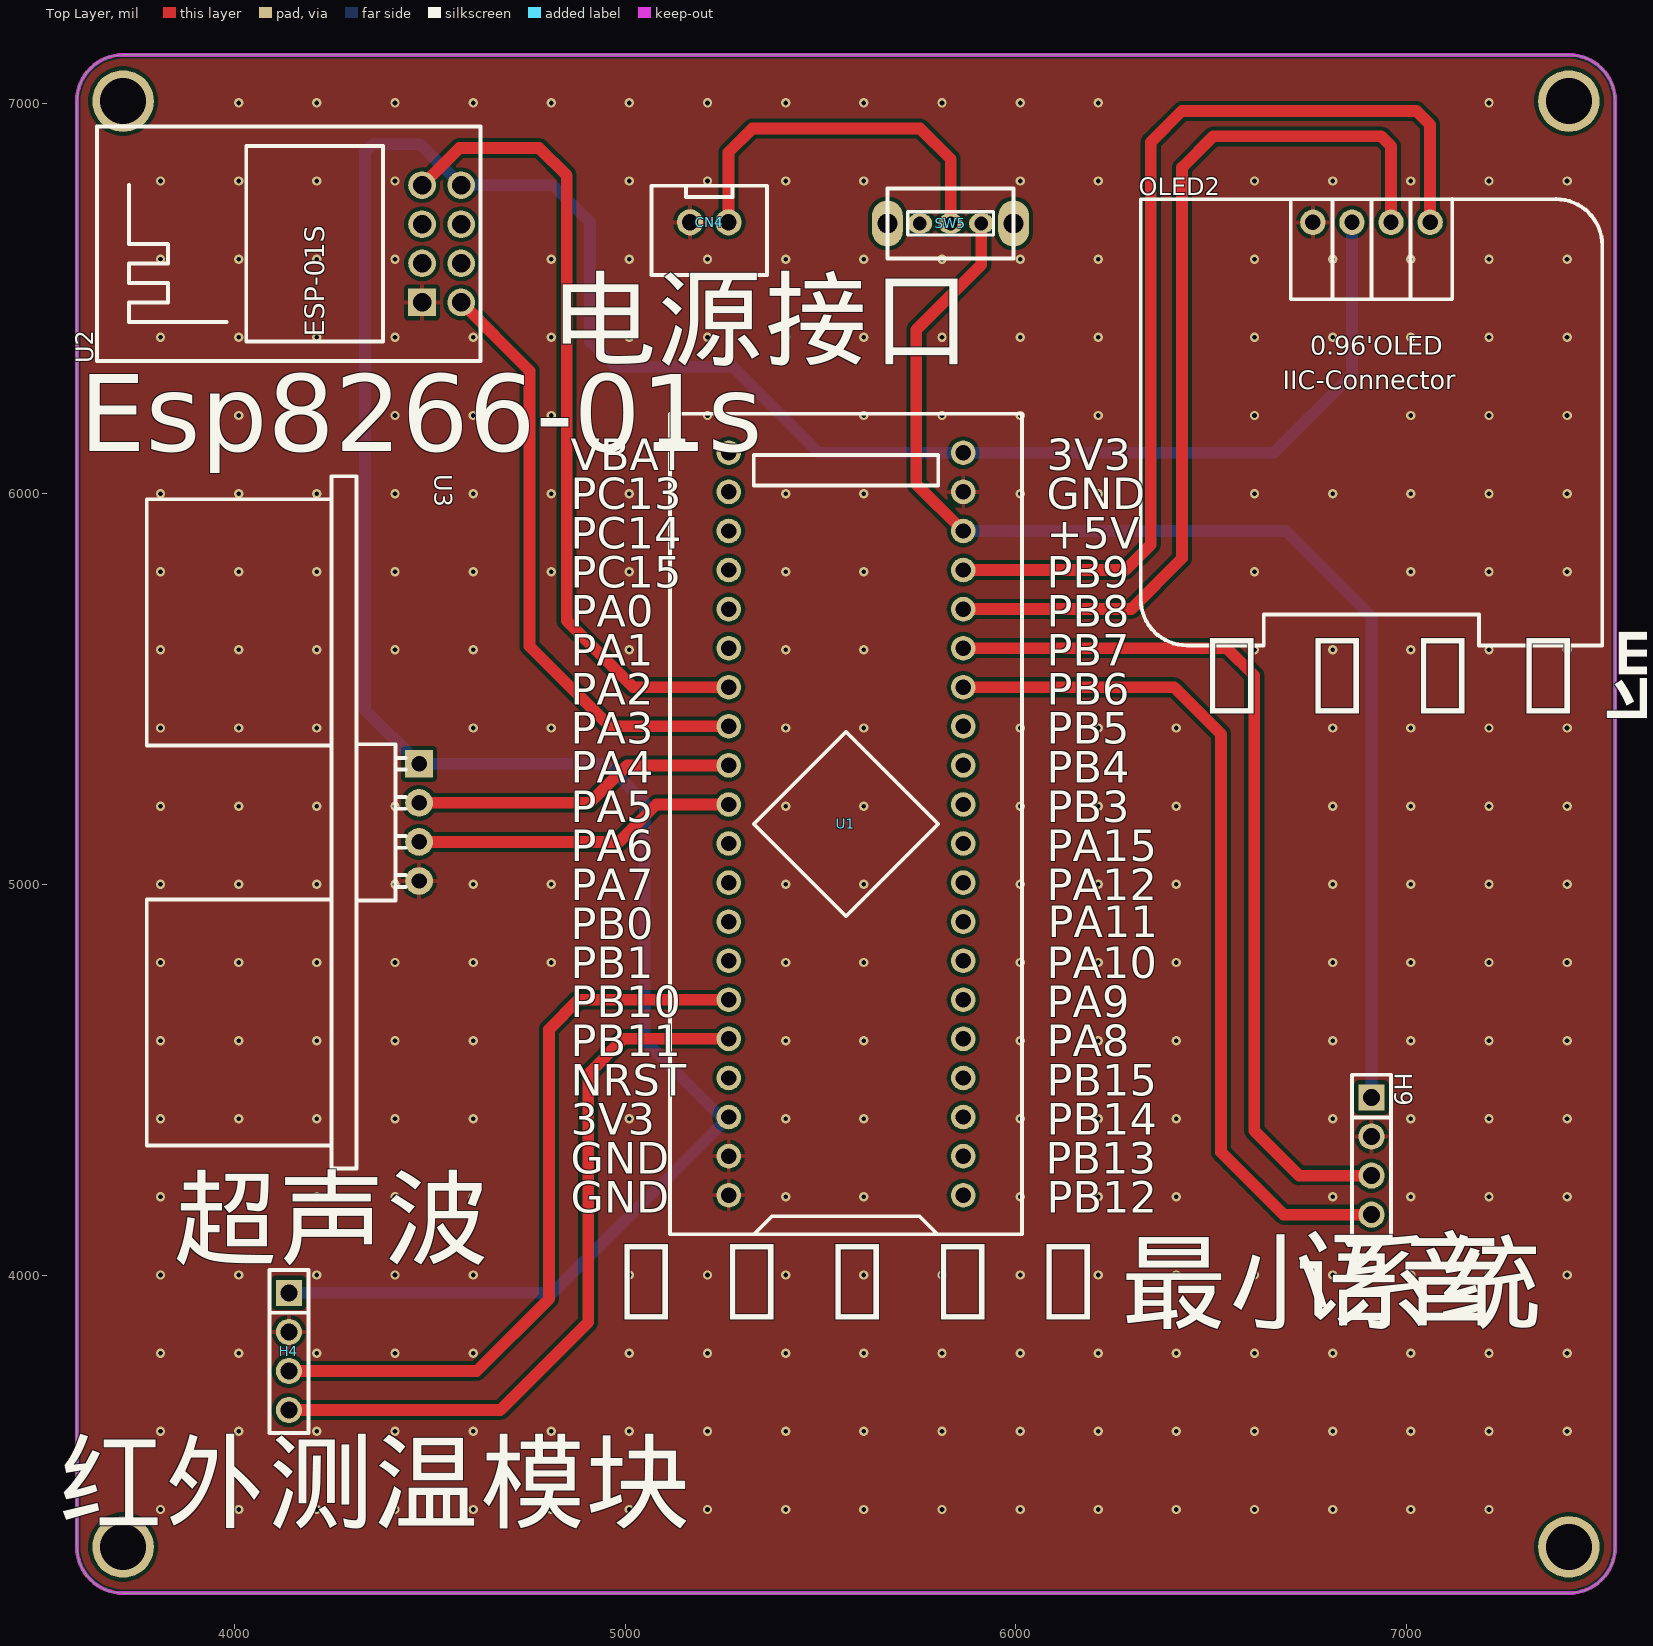
[diagram p0: Top Layer view]
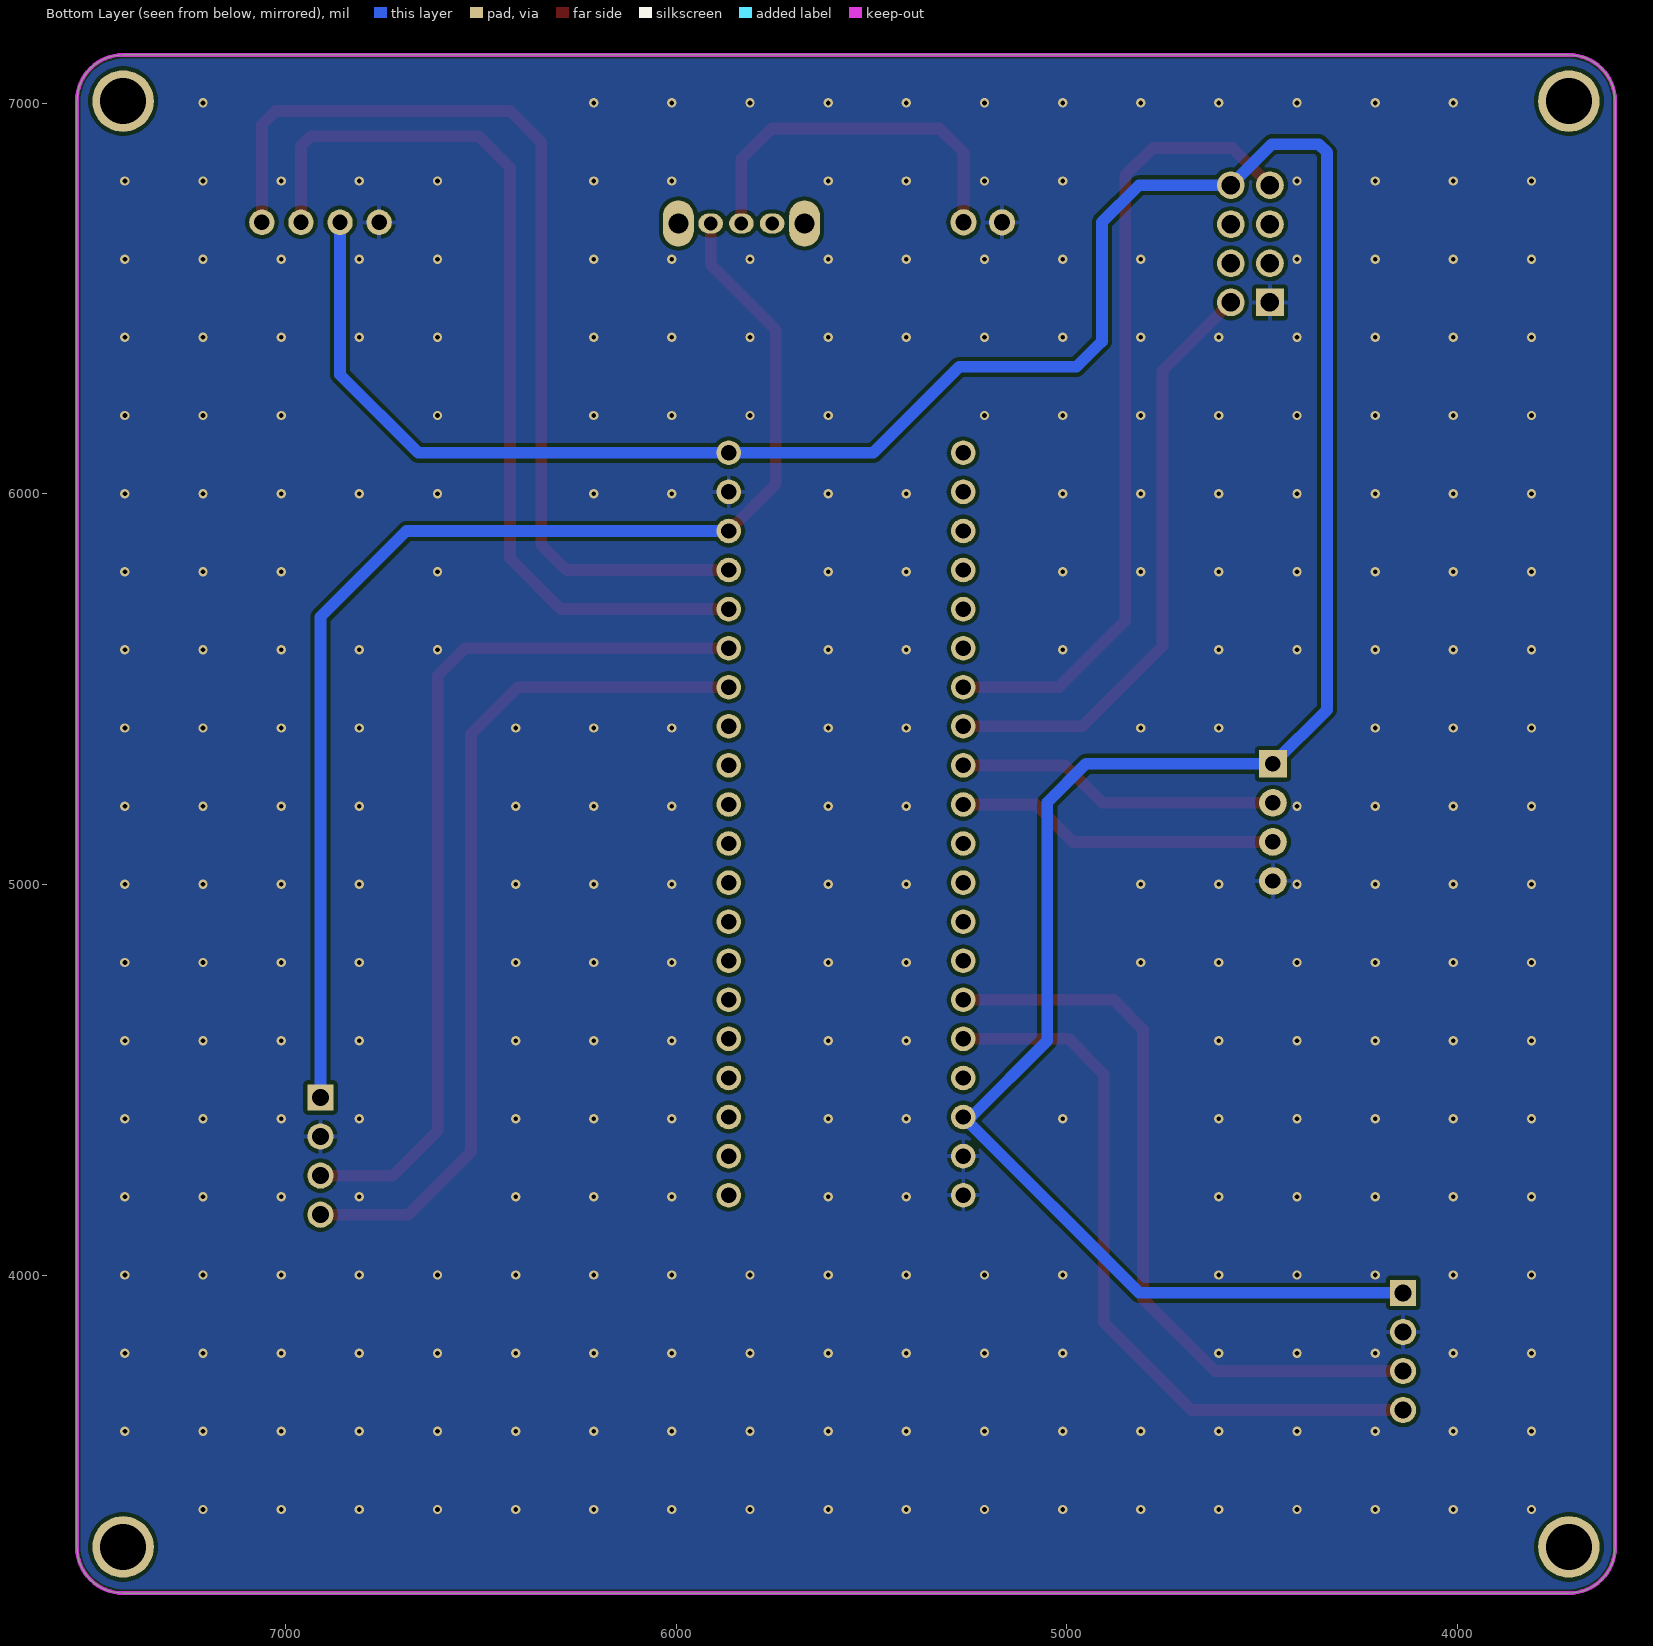
[diagram p1: Bottom Layer view, seen from below]
# Altium PCB MISC51851.pcbdoc
Units mil, origin at the board's own origin, x right, y up, seen from the top; angles counter-clockwise.
Board outline 3937.01 x 3937.01 mil, 2 copper layers (Top Layer, Bottom Layer), stack 62.206 mil thick; 8 components, 38 nets, 75 pads, 294 vias.

## Layer stack, top to bottom
Top Solder Mask Layer: solder mask 0.394, Dk 3.3
Top Layer: signal copper 1.379
Dielectric1: surface 59.449, FR4, Dk 4.5
Bottom Layer: signal copper 1.378
Bottom Solder Mask Layer: solder mask 0.394, Dk 3.3

## Board outline
3714.61,7123.5 ccw(c3714.61,7005.39) 3596.5,7005.39 3596.5,3304.61 ccw(c3714.61,3304.61) 3714.61,3186.5 7415.39,3186.5 ccw(c7415.39,3304.61) 7533.5,3304.61 7533.5,7005.39 ccw(c7415.39,7005.39) 7415.39,7123.5 3714.61,7123.5

## Design rules (kind name [scope] priority, off if disabled: settings)
BoardOutlineClearance copperThickness2oz_1 [All] p2 off: genericclearance=7.99 ignorepadtopadclearanceinfootprint=FALSE except(0: Arc-SplitContinuation Track-SplitContinuation SMDPad-SplitContinuation THPad-SplitContinuation Via-SplitContinuation Fill-SplitContinuation Region-SplitContinuation Poly-SplitContinuation Text-SplitContinuation Hole-SplitContinuation; 5.98: Arc-CutoutEdge Track-CutoutEdge SMDPad-CutoutEdge THPad-CutoutEdge Via-CutoutEdge Text-CutoutEdge; 6.9: Hole-OutlineEdge Hole-CutoutEdge; 10: Poly-OutlineEdge Poly-CutoutEdge; 11.81: Arc-OutlineEdge Track-OutlineEdge SMDPad-OutlineEdge THPad-OutlineEdge Via-OutlineEdge Fill-OutlineEdge Region-OutlineEdge Text-OutlineEdge Fill-CutoutEdge Region-CutoutEdge)
BoardOutlineClearance Plane_innerPlane_1 [All] p4 off: genericclearance=4.02 ignorepadtopadclearanceinfootprint=FALSE except(0: Arc-SplitContinuation Track-SplitContinuation SMDPad-SplitContinuation THPad-SplitContinuation Via-SplitContinuation Fill-SplitContinuation Region-SplitContinuation Poly-SplitContinuation Text-SplitContinuation Hole-SplitContinuation; 5.98: Arc-CutoutEdge Track-CutoutEdge SMDPad-CutoutEdge THPad-CutoutEdge Via-CutoutEdge Text-CutoutEdge; 6.9: Hole-OutlineEdge Hole-CutoutEdge; 10: Poly-OutlineEdge Poly-CutoutEdge; 11.81: Arc-OutlineEdge Track-OutlineEdge SMDPad-OutlineEdge THPad-OutlineEdge Via-OutlineEdge Fill-OutlineEdge Region-OutlineEdge Text-OutlineEdge Fill-CutoutEdge Region-CutoutEdge)
BoardOutlineClearance Copper_copperRegion_1 [All] p6 off: genericclearance=4.02 ignorepadtopadclearanceinfootprint=FALSE except(0: Arc-SplitContinuation Track-SplitContinuation SMDPad-SplitContinuation THPad-SplitContinuation Via-SplitContinuation Fill-SplitContinuation Region-SplitContinuation Poly-SplitContinuation Text-SplitContinuation Hole-SplitContinuation; 5.98: Arc-CutoutEdge Track-CutoutEdge SMDPad-CutoutEdge THPad-CutoutEdge Via-CutoutEdge Text-CutoutEdge; 6.9: Hole-OutlineEdge Hole-CutoutEdge; 10: Poly-OutlineEdge Poly-CutoutEdge; 11.81: Arc-OutlineEdge Track-OutlineEdge SMDPad-OutlineEdge THPad-OutlineEdge Via-OutlineEdge Fill-OutlineEdge Region-OutlineEdge Text-OutlineEdge Fill-CutoutEdge Region-CutoutEdge)
BoardOutlineClearance Copper_copperRegion_copperThickness1oz_1 [All] p8 off: genericclearance=4.02 ignorepadtopadclearanceinfootprint=FALSE except(0: Arc-SplitContinuation Track-SplitContinuation SMDPad-SplitContinuation THPad-SplitContinuation Via-SplitContinuation Fill-SplitContinuation Region-SplitContinuation Poly-SplitContinuation Text-SplitContinuation Hole-SplitContinuation; 5.98: Arc-CutoutEdge Track-CutoutEdge SMDPad-CutoutEdge THPad-CutoutEdge Via-CutoutEdge Text-CutoutEdge; 6.9: Hole-OutlineEdge Hole-CutoutEdge; 10: Poly-OutlineEdge Poly-CutoutEdge; 11.81: Arc-OutlineEdge Track-OutlineEdge SMDPad-OutlineEdge THPad-OutlineEdge Via-OutlineEdge Fill-OutlineEdge Region-OutlineEdge Text-OutlineEdge Fill-CutoutEdge Region-CutoutEdge)
BoardOutlineClearance Copper_copperRegion_Copper_copperRegion_1 [All] p10 off: genericclearance=4.02 ignorepadtopadclearanceinfootprint=FALSE except(0: Arc-SplitContinuation Track-SplitContinuation SMDPad-SplitContinuation THPad-SplitContinuation Via-SplitContinuation Fill-SplitContinuation Region-SplitContinuation Poly-SplitContinuation Text-SplitContinuation Hole-SplitContinuation; 5.98: Arc-CutoutEdge Track-CutoutEdge SMDPad-CutoutEdge THPad-CutoutEdge Via-CutoutEdge Text-CutoutEdge; 6.9: Hole-OutlineEdge Hole-CutoutEdge; 10: Poly-OutlineEdge Poly-CutoutEdge; 11.81: Arc-OutlineEdge Track-OutlineEdge SMDPad-OutlineEdge THPad-OutlineEdge Via-OutlineEdge Fill-OutlineEdge Region-OutlineEdge Text-OutlineEdge Fill-CutoutEdge Region-CutoutEdge)
BoardOutlineClearance copperThickness1oz_1 [All] p12: genericclearance=4.02 ignorepadtopadclearanceinfootprint=FALSE except(0: Arc-SplitContinuation Track-SplitContinuation SMDPad-SplitContinuation THPad-SplitContinuation Via-SplitContinuation Fill-SplitContinuation Region-SplitContinuation Poly-SplitContinuation Text-SplitContinuation Hole-SplitContinuation; 5.98: Arc-CutoutEdge Track-CutoutEdge SMDPad-CutoutEdge THPad-CutoutEdge Via-CutoutEdge Text-CutoutEdge; 6.9: Hole-OutlineEdge Hole-CutoutEdge; 10: Poly-OutlineEdge Poly-CutoutEdge; 11.81: Arc-OutlineEdge Track-OutlineEdge SMDPad-OutlineEdge THPad-OutlineEdge Via-OutlineEdge Fill-OutlineEdge Region-OutlineEdge Text-OutlineEdge Fill-CutoutEdge Region-CutoutEdge)
Clearance copperThickness2oz [All] p1 off: gap=7.99 ignorepadtopadclearanceinfootprint=FALSE except(5.98: SMDPad-Track SMDPad-SMDPad THPad-Track SMDPad-THPad THPad-THPad Track-Via SMDPad-Via THPad-Via Via-Via Fill-SMDPad Region-SMDPad Fill-THPad Region-THPad Fill-Via Region-Via Fill-Fill Fill-Region Region-Region Arc-Track Arc-SMDPad Arc-THPad Arc-Via Fill-Arc Region-Arc Arc-Arc Text-Track SMDPad-Text Text-THPad Text-Via Fill-Text Region-Text Arc-Text Text-Text; 6.9: Hole-Track Hole-SMDPad Hole-THPad Hole-Via Fill-Hole Region-Hole Hole-Arc Hole-Text; 10: Poly-Track Poly-SMDPad Poly-THPad Poly-Via Poly-Fill Poly-Region Poly-Poly Poly-Arc Poly-Text Poly-Hole; 11.81: Fill-Track Region-Track)
Clearance Plane_innerPlane [All] p3 off: gap=4.02 ignorepadtopadclearanceinfootprint=FALSE except(5.98: SMDPad-Track SMDPad-SMDPad THPad-Track SMDPad-THPad THPad-THPad Track-Via SMDPad-Via THPad-Via Via-Via Fill-SMDPad Region-SMDPad Fill-THPad Region-THPad Fill-Via Region-Via Fill-Fill Fill-Region Region-Region Arc-Track Arc-SMDPad Arc-THPad Arc-Via Fill-Arc Region-Arc Arc-Arc Text-Track SMDPad-Text Text-THPad Text-Via Fill-Text Region-Text Arc-Text Text-Text; 6.9: Hole-Track Hole-SMDPad Hole-THPad Hole-Via Fill-Hole Region-Hole Hole-Arc Hole-Text; 10: Poly-Track Poly-SMDPad Poly-THPad Poly-Via Poly-Fill Poly-Region Poly-Poly Poly-Arc Poly-Text Poly-Hole; 11.81: Fill-Track Region-Track)
Clearance Copper_copperRegion [All] p5 off: gap=4.02 ignorepadtopadclearanceinfootprint=FALSE except(5.98: SMDPad-Track SMDPad-SMDPad THPad-Track SMDPad-THPad THPad-THPad Track-Via SMDPad-Via THPad-Via Via-Via Fill-SMDPad Region-SMDPad Fill-THPad Region-THPad Fill-Via Region-Via Fill-Fill Fill-Region Region-Region Arc-Track Arc-SMDPad Arc-THPad Arc-Via Fill-Arc Region-Arc Arc-Arc Text-Track SMDPad-Text Text-THPad Text-Via Fill-Text Region-Text Arc-Text Text-Text; 6.9: Hole-Track Hole-SMDPad Hole-THPad Hole-Via Fill-Hole Region-Hole Hole-Arc Hole-Text; 10: Poly-Track Poly-SMDPad Poly-THPad Poly-Via Poly-Fill Poly-Region Poly-Poly Poly-Arc Poly-Text Poly-Hole; 11.81: Fill-Track Region-Track)
Clearance Copper_copperRegion_copperThickness1oz [All] p7 off: gap=4.02 ignorepadtopadclearanceinfootprint=FALSE except(5.98: SMDPad-Track SMDPad-SMDPad THPad-Track SMDPad-THPad THPad-THPad Track-Via SMDPad-Via THPad-Via Via-Via Fill-SMDPad Region-SMDPad Fill-THPad Region-THPad Fill-Via Region-Via Fill-Fill Fill-Region Region-Region Arc-Track Arc-SMDPad Arc-THPad Arc-Via Fill-Arc Region-Arc Arc-Arc Text-Track SMDPad-Text Text-THPad Text-Via Fill-Text Region-Text Arc-Text Text-Text; 6.9: Hole-Track Hole-SMDPad Hole-THPad Hole-Via Fill-Hole Region-Hole Hole-Arc Hole-Text; 10: Poly-Track Poly-SMDPad Poly-THPad Poly-Via Poly-Fill Poly-Region Poly-Poly Poly-Arc Poly-Text Poly-Hole; 11.81: Fill-Track Region-Track)
Clearance Copper_copperRegion_Copper_copperRegion [All] p9 off: gap=4.02 ignorepadtopadclearanceinfootprint=FALSE except(5.98: SMDPad-Track SMDPad-SMDPad THPad-Track SMDPad-THPad THPad-THPad Track-Via SMDPad-Via THPad-Via Via-Via Fill-SMDPad Region-SMDPad Fill-THPad Region-THPad Fill-Via Region-Via Fill-Fill Fill-Region Region-Region Arc-Track Arc-SMDPad Arc-THPad Arc-Via Fill-Arc Region-Arc Arc-Arc Text-Track SMDPad-Text Text-THPad Text-Via Fill-Text Region-Text Arc-Text Text-Text; 6.9: Hole-Track Hole-SMDPad Hole-THPad Hole-Via Fill-Hole Region-Hole Hole-Arc Hole-Text; 10: Poly-Track Poly-SMDPad Poly-THPad Poly-Via Poly-Fill Poly-Region Poly-Poly Poly-Arc Poly-Text Poly-Hole; 11.81: Fill-Track Region-Track)
Clearance copperThickness1oz [All] p11: gap=4.02 ignorepadtopadclearanceinfootprint=FALSE except(5.98: SMDPad-Track SMDPad-SMDPad THPad-Track SMDPad-THPad THPad-THPad Track-Via SMDPad-Via THPad-Via Via-Via Fill-SMDPad Region-SMDPad Fill-THPad Region-THPad Fill-Via Region-Via Fill-Fill Fill-Region Region-Region Arc-Track Arc-SMDPad Arc-THPad Arc-Via Fill-Arc Region-Arc Arc-Arc Text-Track SMDPad-Text Text-THPad Text-Via Fill-Text Region-Text Arc-Text Text-Text; 6.9: Hole-Track Hole-SMDPad Hole-THPad Hole-Via Fill-Hole Region-Hole Hole-Arc Hole-Text; 10: Poly-Track Poly-SMDPad Poly-THPad Poly-Via Poly-Fill Poly-Region Poly-Poly Poly-Arc Poly-Text Poly-Hole; 11.81: Fill-Track Region-Track)
DiffPairsRouting differentialPair [All] p1: maxlimit=6 minlimit=6 mostfreqgap=6 toplayer_minwidth=5 toplayer_prefwidth=10 toplayer_maxwidth=100 toplayer_mingap=6 toplayer_prefgap=6 toplayer_maxgap=6 bottomlayer_minwidth=5 bottomlayer_prefwidth=10 bottomlayer_maxwidth=100 bottomlayer_mingap=6 bottomlayer_prefgap=6 bottomlayer_maxgap=6 maxuncoupledlength=10
HoleToHoleClearance otherClearance [All] p1: gap=11.81 allowstackedmicrovias=TRUE
Length netLength [All] p1: minlimit=0 maxlimit=0
PasteMaskExpansion pasteMaskExpansion [All] p1: expansion=0
PlaneConnect innerPlane [All] p1: planeconnectstyle=Relief reliefexpansion=20 reliefentries=4 reliefconductorwidth=10 reliefairgap=10
PolygonConnect copperRegion_copperThickness1oz [All] p1 off: connectstyle=Relief reliefconductorwidth=10 reliefentries=4 polygonreliefangle="90 Angle" airgapwidth=10 via.connectstyle=Relief via.reliefconductorwidth=10 via.reliefentries=4 via.polygonreliefangle="90 Angle" via.airgapwidth=10
PolygonConnect copperRegion_Copper_copperRegion [All] p2 off: connectstyle=Relief reliefconductorwidth=10 reliefentries=4 polygonreliefangle="90 Angle" airgapwidth=10 via.connectstyle=Relief via.reliefconductorwidth=10 via.reliefentries=4 via.polygonreliefangle="90 Angle" via.airgapwidth=10
PolygonConnect copperRegion [All] p3: connectstyle=Relief reliefconductorwidth=10 reliefentries=4 polygonreliefangle="90 Angle" airgapwidth=10 via.connectstyle=Relief via.reliefconductorwidth=10 via.reliefentries=4 via.polygonreliefangle="90 Angle" via.airgapwidth=10
RoutingVias viaSize [All] p1: holewidth=12.01 width=24.02 viastyle="Through Hole" minholewidth=11.81 minwidth=19.68 maxholewidth=248.03 maxwidth=393.7
SolderMaskExpansion solderMaskExpansion [IsVia] p1: expansion=-1000 istentingtop=TRUE
SolderMaskExpansion solderMaskExpansion [All] p2: expansion=2 istentingtop=FALSE
Width copperThickness2oz_2 [All] p1 off: maxlimit=100 minlimit=8 preferedwidth=10
Width copperThickness1oz_2 [All] p2: maxlimit=100 minlimit=5 preferedwidth=10

## Components (designator, comment, footprint, x,y, rotation, side; value= is the part's Value field where it differs from the comment)
CN4 "XH2.54*2P_直插" CONN-TH_2P-P2.50-XH2.54-2P 5215,6695 r0 top
H4 "" HDR-TH_4P-P2.54-V-F 4139,3804.93 r270 top
H9 "" HDR-TH_4P-P2.54-V-F 6910,4305 r270 top
OLED2 "" 0.96OLED_4P 6910,6695 r0 top
SW5 "" 拨动开关 5837.9,6692.05 r180 top
U1 "STM32F103C8T6-Card" CONN-TH_L53.3-W22.9_STM32F103C8T6-CARD 5565,5155 r90 top
U2 "ESP-01S" WIFIM-TH_ESP-01S 4530,6640 r90 top
U3 "HC-SR04" TH_HC-SR04V 4472.28,5159.1 r270 top

## Footprints (in the part's own frame and the unit in brackets; to place one, negate y for a bottom-side part, rotate by r counter-clockwise, add the part's x,y. Pads: shape width x height; smd on the part's side, far side on the other; paste and mask are expansions set on the pad)
0.96OLED_4P [mm]
  round 1.65 hole 1 copper offset 0,0: 1(-3.81,-0.001) 2(-1.27,0.002) 3(1.27,0.002) 4(3.81,0.002)
  silkscreen extent -15,-27.5 15,1.5
CONN-TH_2P-P2.50-XH2.54-2P [mm]
  round 1.7 hole 1.05 paste+0 mask+0.05: 1(1.25,0) 2(-1.25,0)
  silkscreen extent -3.75,-3.42 3.75,2.37
CONN-TH_L53.3-W22.9_STM32F103C8T6-CARD [mm]
  round 1.6 hole 1: 1(-24.13,-7.62) 2(-21.59,-7.62) 3(-19.05,-7.62) 4(-16.51,-7.62) 5(-13.97,-7.62) 6(-11.43,-7.62) 7(-8.89,-7.62) 8(-6.35,-7.62) 9(-3.81,-7.62) 10(-1.27,-7.62) 11(1.27,-7.62) 12(3.81,-7.62) 13(6.35,-7.62) 14(8.89,-7.62) 15(11.43,-7.62) 16(13.97,-7.62) 17(16.51,-7.62) 18(19.05,-7.62) 19(21.59,-7.62) 20(24.13,-7.62) 21(24.13,7.62) 22(21.59,7.62) 23(19.05,7.62) 24(16.51,7.62) 25(13.97,7.62) 26(11.43,7.62) 27(8.89,7.62) 28(6.35,7.62) 29(3.81,7.62) 30(1.27,7.62) 31(-1.27,7.62) 32(-3.81,7.62) 33(-6.35,7.62) 34(-8.89,7.62) 35(-11.43,7.62) 36(-13.97,7.62) 37(-16.51,7.62) 38(-19.05,7.62) 39(-21.59,7.62) 40(-24.13,7.62)
  silkscreen extent -26.67,-11.43 26.67,11.43
HDR-TH_4P-P2.54-V-F [mm]
  rect 1.7x1.7 hole 1.1: 1(-3.81,0)
  round 1.7 hole 1.1: 2(-1.27,0) 3(1.27,0) 4(3.81,0)
  silkscreen extent -5.29,-1.27 5.29,1.27
TH_HC-SR04V [mm]
  rect 1.8x1.8 hole 1.001: 1(-3.81,0)
  round 1.8 hole 1.001: 2(-1.27,0) 3(1.27,0) 4(3.81,0)
  silkscreen extent -22.5,-17.7 22.5,-0.89
WIFIM-TH_ESP-01S [mm]
  rect 1.8x1.8 hole 1.2: 1(-3.81,1.27)
  round 1.8 hole 1.2: 2(-1.27,1.27) 3(1.27,1.27) 4(3.81,1.27) 5(3.81,-1.27) 6(1.27,-1.27) 7(-1.27,-1.27) 8(-3.81,-1.27)
  silkscreen extent -7.62,-2.54 7.62,22.4
拨动开关 [mil]
  oval 63x51.2 hole 35.4 paste+0 mask+2: 1(-73.4,0) 2(5,0) 3(84,0)
  oval 78.7x118.1 hole 51.2 paste+0 mask+2: 4(166.7,0) 5(-156.1,0)
  silkscreen extent -156,-90 167,90

## Free pads (board coordinates)
  round 157.48 hole 118.11: 1(3714.61,7005.39) 1(3714.61,3304.61) 1(7415.39,7005.39) 1(7415.39,3304.61)

## Via types
v1: diameter 24.02, hole 12, Top Layer to Bottom Layer, 294 vias

## Nets (pads, with @x,y where several pads share a name; then routed paths per layer and width w, separated by ;. In a path a pad name is that pad's centre, name@x,y a point inside that pad or via, vN(x,y) a via of type N, cw(c..) or ccw(c..) an arc to the next point about the centre after c; other vN are vias at no path point)
$1N17118: CN4.1 SW5.2 | length 970.4
  Top Layer w30: CN4.1 5264.22,6874.22 5325,6935 5755,6935 5832.9,6857.1 SW5.2
+5V: H9.1 SW5.1 U1.18 | length 3271.8
  Top Layer w30: U1.18 5745,6025 5745,6420 5911.3,6586.3 SW5.1
  Bottom Layer w30: U1.18 6690,5905 6910,5685 H9.1
GND: CN4.2 H4.2 H9.2 OLED2.1 U1.19 U1.39 U1.40 U2.1 U3.4
  other v1: 3810.6,3400.6 4010.6,3400.6 4210.6,3400.6 4410.6,3400.6 4610.6,3400.6 4810.6,3400.6 5010.6,3400.6 5210.6,3400.6 5410.6,3400.6 5610.6,3400.6 5810.6,3400.6 6010.6,3400.6 6210.6,3400.6 6410.6,3400.6 6610.6,3400.6 6810.6,3400.6 7010.6,3400.6 7210.6,3400.6 3810.6,3600.6 4010.6,3600.6 4210.6,3600.6 4410.6,3600.6 4610.6,3600.6 4810.6,3600.6 5010.6,3600.6 5210.6,3600.6 5410.6,3600.6 5610.6,3600.6 5810.6,3600.6 6010.6,3600.6 6210.6,3600.6 6410.6,3600.6 6610.6,3600.6 6810.6,3600.6 7010.6,3600.6 7210.6,3600.6 7410.6,3600.6 3810.6,3800.6 4010.6,3800.6 4210.6,3800.6 4410.6,3800.6 4610.6,3800.6 5010.6,3800.6 5210.6,3800.6 5410.6,3800.6 5610.6,3800.6 5810.6,3800.6 6010.6,3800.6 6210.6,3800.6 6410.6,3800.6 6610.6,3800.6 6810.6,3800.6 7010.6,3800.6 7210.6,3800.6 7410.6,3800.6 3810.6,4000.6 4010.6,4000.6 4210.6,4000.6 4410.6,4000.6 4610.6,4000.6 5010.6,4000.6 5210.6,4000.6 5410.6,4000.6 5610.6,4000.6 5810.6,4000.6 6010.6,4000.6 6210.6,4000.6 6410.6,4000.6 6610.6,4000.6 6810.6,4000.6 7010.6,4000.6 7210.6,4000.6 7410.6,4000.6 3810.6,4200.6 4010.6,4200.6 4210.6,4200.6 4410.6,4200.6 4610.6,4200.6 5410.6,4200.6 5610.6,4200.6 6010.6,4200.6 6210.6,4200.6 6410.6,4200.6 6810.6,4200.6 7010.6,4200.6 7210.6,4200.6 7410.6,4200.6 3810.6,4400.6 4010.6,4400.6 4210.6,4400.6 4410.6,4400.6 4610.6,4400.6 5010.6,4400.6 5410.6,4400.6 5610.6,4400.6 6010.6,4400.6 6210.6,4400.6 6410.6,4400.6 6810.6,4400.6 7010.6,4400.6 7210.6,4400.6 7410.6,4400.6 3810.6,4600.6 4010.6,4600.6 4210.6,4600.6 4410.6,4600.6 4610.6,4600.6 5410.6,4600.6 5610.6,4600.6 6010.6,4600.6 6210.6,4600.6 6410.6,4600.6 6810.6,4600.6 7010.6,4600.6 7210.6,4600.6 7410.6,4600.6 3810.6,4800.6 4010.6,4800.6 4210.6,4800.6 4410.6,4800.6 4610.6,4800.6 4810.6,4800.6 5410.6,4800.6 5610.6,4800.6 6010.6,4800.6 6210.6,4800.6 6410.6,4800.6 6810.6,4800.6 7010.6,4800.6 7210.6,4800.6 7410.6,4800.6 3810.6,5000.6 4010.6,5000.6 4210.6,5000.6 4410.6,5000.6 4610.6,5000.6 4810.6,5000.6 5410.6,5000.6 5610.6,5000.6 6010.6,5000.6 6210.6,5000.6 6410.6,5000.6 6810.6,5000.6 7010.6,5000.6 7210.6,5000.6 7410.6,5000.6 3810.6,5200.6 4010.6,5200.6 4210.6,5200.6 4410.6,5200.6 5410.6,5200.6 5610.6,5200.6 6010.6,5200.6 6210.6,5200.6 6410.6,5200.6 6810.6,5200.6 7010.6,5200.6 7210.6,5200.6 7410.6,5200.6 3810.6,5400.6 4010.6,5400.6 4210.6,5400.6 4610.6,5400.6 4810.6,5400.6 5410.6,5400.6 5610.6,5400.6 6010.6,5400.6 6210.6,5400.6 6410.6,5400.6 6810.6,5400.6 7010.6,5400.6 7210.6,5400.6 7410.6,5400.6 3810.6,5600.6 4010.6,5600.6 4210.6,5600.6 4410.6,5600.6 4610.6,5600.6 5010.6,5600.6 5410.6,5600.6 5610.6,5600.6 6610.6,5600.6 6810.6,5600.6 7010.6,5600.6 7210.6,5600.6 7410.6,5600.6 3810.6,5800.6 4010.6,5800.6 4210.6,5800.6 4410.6,5800.6 4610.6,5800.6 4810.6,5800.6 5010.6,5800.6 5410.6,5800.6 5610.6,5800.6 6610.6,5800.6 7010.6,5800.6 7210.6,5800.6 7410.6,5800.6 3810.6,6000.6 4010.6,6000.6 4210.6,6000.6 4410.6,6000.6 4610.6,6000.6 4810.6,6000.6 5010.6,6000.6 5410.6,6000.6 5610.6,6000.6 6010.6,6000.6 6210.6,6000.6 6610.6,6000.6 6810.6,6000.6 7010.6,6000.6 7210.6,6000.6 7410.6,6000.6 3810.6,6200.6 4010.6,6200.6 4210.6,6200.6 4410.6,6200.6 4610.6,6200.6 4810.6,6200.6 5010.6,6200.6 5210.6,6200.6 5610.6,6200.6 5810.6,6200.6 6010.6,6200.6 6210.6,6200.6 6610.6,6200.6 7010.6,6200.6 7210.6,6200.6 7410.6,6200.6 3810.6,6400.6 4010.6,6400.6 4210.6,6400.6 4410.6,6400.6 4610.6,6400.6 4810.6,6400.6 5010.6,6400.6 5210.6,6400.6 5410.6,6400.6 5610.6,6400.6 5810.6,6400.6 6010.6,6400.6 6210.6,6400.6 6610.6,6400.6 6810.6,6400.6 7010.6,6400.6 7210.6,6400.6 7410.6,6400.6 3810.6,6600.6 4010.6,6600.6 4210.6,6600.6 4410.6,6600.6 4810.6,6600.6 5010.6,6600.6 5210.6,6600.6 5410.6,6600.6 5610.6,6600.6 5810.6,6600.6 6010.6,6600.6 6210.6,6600.6 6610.6,6600.6 6810.6,6600.6 7010.6,6600.6 7210.6,6600.6 7410.6,6600.6 3810.6,6800.6 4010.6,6800.6 4210.6,6800.6 4410.6,6800.6 5010.6,6800.6 5210.6,6800.6 5410.6,6800.6 5610.6,6800.6 6010.6,6800.6 6210.6,6800.6 6610.6,6800.6 6810.6,6800.6 7010.6,6800.6 7210.6,6800.6 7410.6,6800.6 4010.6,7000.6 4210.6,7000.6 4410.6,7000.6 4610.6,7000.6 4810.6,7000.6 5010.6,7000.6 5210.6,7000.6 5410.6,7000.6 5610.6,7000.6 5810.6,7000.6 6010.6,7000.6 6210.6,7000.6 7210.6,7000.6
NRST: U1.37
PA0: U1.25
PA1: U1.26
PA2: U1.27 U2.4 | length 2063.8
  Top Layer w30: U2.4 4575,6885 4780,6885 4850,6815 4850,5675 5020,5505 U1.27
PA3: U1.28 U2.8 | length 1547.4
  Top Layer w30: U2.8 4755,6315 4755,5610 4960,5405 U1.28
PA4: U1.29 U3.2 | length 832.4
  Top Layer w30: U3.2 4909.1,5209.1 5005,5305 U1.29
PA5: U1.30 U3.3 | length 832.4
  Top Layer w30: U3.3 4984.1,5109.1 5080,5205 U1.30
PA6: U1.31
PA7: U1.32
PA8: U1.5
PA9: U1.6
PA10: U1.7
PA11: U1.8
PA12: U1.9
PA15: U1.10
PB0: U1.33
PB1: U1.34
PB3: U1.11
PB4: U1.12
PB5: U1.13
PB6: H9.4 U1.14 | length 2231
  Top Layer w30: U1.14 6405,5505 6525,5385 6525,4315 6685,4155 H9.4
PB7: H9.3 U1.15 | length 2286.6
  Top Layer w30: U1.15 6540,5605 6610,5535 6610,4370 6725,4255 H9.3
PB8: OLED2.3 U1.16 | length 2387.3
  Top Layer w30: U1.16 6295,5705 6425,5835 6425,6835 6505,6915 6935,6915 6960,6890 OLED2.3@6960,6695.05
PB9: OLED2.4 U1.17 | length 2549.5
  Top Layer w30: U1.17 6280,5805 6345,5870 6345,6900 6425,6980 7025,6980 7060,6945 OLED2.4@7060,6695.05
PB10: H4.3 U1.35 | length 1923.7
  Top Layer w30: H4.3 4619.93,3754.93 4805,3940 4805,4630 4880,4705 U1.35
PB11: H4.4 U1.36 | length 1891.5
  Top Layer w30: H4.4 4679.93,3654.93 4905,3880 4905,4515 4995,4605 U1.36
PB12: U1.1
PB13: U1.2
PB14: U1.3
PB15: U1.4
PC13: U1.22
PC14: U1.23
PC15: U1.24
VBAT: U1.21
VCC: H4.1 OLED2.2 U1.20 U1.38 U2.5 U3.1 | length 7972.8
  Bottom Layer w30: H4.1 4814.93,3954.93 U1.38 5245,4405 5050,4600 5050,5210 4950.9,5309.1 U3.1 4333.79,5447.6 4333.79,6873.79 4355,6895 4475,6895 U2.5 4815,6790 4910,6695 4910,6390 4975,6325 5275,6325 5495,6105 U1.20 6660,6105 6860,6305 OLED2.2@6860,6695.05
pads on no net: SW5.3 SW5.4 SW5.5 U2.2 U2.3 U2.6 U2.7

## Polygon pours and split planes (outlines as drawn)
GND on Bottom Layer (solid, remove dead copper, pour order 2): 3525,7245 3525,3080 7700,3080 7700,7245
GND on Top Layer (solid, remove dead copper, pour order 2): 3000,7415 3000,3000 7930,3000 7930,7415

## Keep-outs
Board Outline Layer:
  the board outline again, w10

## Silkscreen, mask and mechanical layers (free items; w line width, h text height)
Top Silkscreen Layer:
  text "电源接口" at 4812.87,6351.57 h196.85
  text "Esp8266-01s" at 3602.14,6108.99 h196.85
  text "VBAT" at 4860.95,6060 h80
  text "3V3" at 6079.16,6060 h80
  text "PC13" at 4860.95,5960 h80
  text "GND" at 6079.16,5960 h80
  text "PC14" at 4860.95,5860 h80
  text "+5V" at 6079.16,5860 h80
  text "PC15" at 4860.95,5760 h80
  text "PB9" at 6079.16,5760 h80
  text "PA0" at 4860.95,5660 h80
  text "PB8" at 6079.16,5660 h80
  text "PA1" at 4860.95,5560 h80
  text "PB7" at 6079.16,5560 h80
  text "PA2" at 4860.95,5460 h80
  text "PB6" at 6079.16,5460 h80
  text "Oled显示器" at 6418.02,5436.57 h196.85
  text "PA3" at 4860.95,5360 h80
  text "PB5" at 6079.16,5360 h80
  text "PA4" at 4860.95,5260 h80
  text "PB4" at 6079.16,5260 h80
  text "PA5" at 4860.95,5160 h80
  text "PB3" at 6079.16,5160 h80
  text "PA6" at 4860.95,5060 h80
  text "PA15" at 6079.16,5060 h80
  text "PA7" at 4860.95,4960 h80
  text "PA12" at 6079.16,4960 h80
  text "PA11" at 6080.95,4865 h80
  text "PB0" at 4860.95,4860 h80
  text "PB1" at 4860.95,4760 h80
  text "PA10" at 6079.16,4760 h80
  text "PB10" at 4860.95,4660 h80
  text "PA9" at 6079.16,4660 h80
  text "PB11" at 4860.95,4560 h80
  text "PA8" at 6079.16,4560 h80
  text "NRST" at 4860.95,4460 h80
  text "PB15" at 6079.16,4460 h80
  text "3V3" at 4860.95,4360 h80
  text "PB14" at 6079.16,4360 h80
  text "GND" at 4860.95,4260 h80
  text "PB13" at 6075.95,4260 h80
  text "GND" at 4860.95,4160 h80
  text "PB12" at 6079.16,4160 h80
  text "超声波" at 3843.72,4051.74 h196.85
  text "语音" at 6713.74,3895 h196.85
  text "STM32最小系统" at 4919.45,3886.57 h196.85
  text "红外测温模块" at 3547.74,3375 h196.85